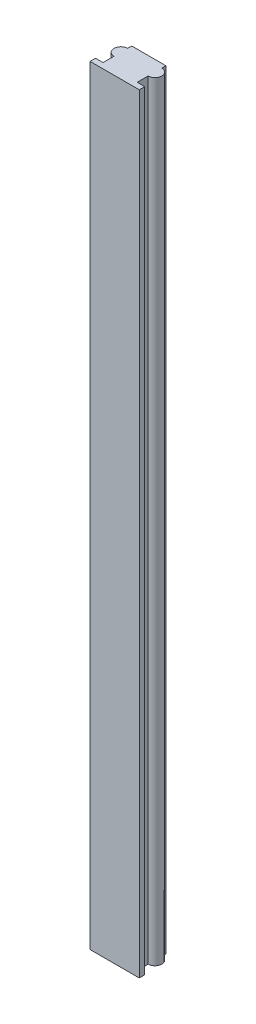
SolidWorks part; units mm, degrees
ref_plane "前视基准面" through (0, 0, 0) normal (0, 0, 1) x (1, 0, 0)
ref_plane "上视基准面" through (0, 0, 0) normal (0, 1, 0) x (1, 0, 0)
ref_plane "右视基准面" through (0, 0, 0) normal (1, 0, 0) x (0, 0, -1)
sketch "草图1" plane through (0, 0, 0) normal (0, 1, 0) x (1, 0, 0)
  line L0 (0, 0) -> (0, 11.3364) construction
  line L1 (-12.5, 5) -> (-12.5, 8)
  line L2 (-12.5, 8) -> (12.5, 8)
  line L3 (12.5, 8) -> (12.5, 5)
  line L4 (-12.5, -5) -> (-12.5, -13)
  line L5 (-12.5, -13) -> (-18, -13)
  line L6 (-18, -13) -> (-18, -17)
  line L7 (-18, -17) -> (18, -17)
  line L8 (18, -17) -> (18, -13)
  line L9 (18, -13) -> (12.5, -13)
  line L10 (12.5, -13) -> (12.5, -5)
  arc A0 (-12.5, 5) -> (-12.5, -5) centre (-12.5, 0) ccw
  arc A1 (12.5, -5) -> (12.5, 5) centre (12.5, 0) ccw
  dimension "D1" = 10
  dimension "D3" = 36
  dimension "D2" = 25
  dimension "D4" = 17
  dimension "D5" = 25
  dimension "D6" = 4
extrude "凸台-拉伸1" add sketch "草图1" along normal blind 563
ref_plane "基准面1" through (0, 0, 0) normal (0, 0, 1) x (1, 0, 0)
